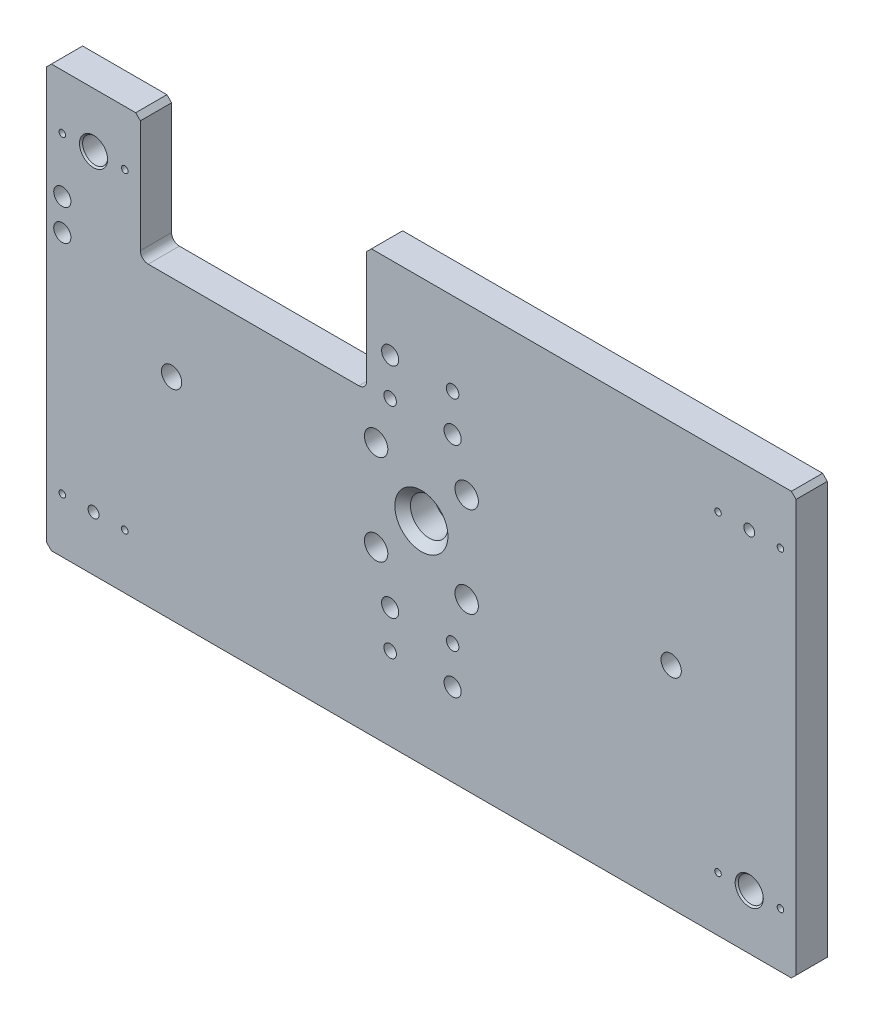
from build123d import *

# Parameters (mm, degrees)
BOSS_EXTRUDE1_DEPTH   = 20
FILLET1_R             = 5
CHAMFER1_SIZE         = 3
HOLE2_D               = 6.6
HOLE2_CBORE_D         = 11
HOLE2_CBORE_DEPTH     = 9
M5_TAPPED_HOLE1_D     = 4.2
M5_TAPPED_HOLE1_DEPTH = 10
M5_TAPPED_HOLE1_TIP   = 1.2618073
M8X1_0_TAPPED_HOLE1_D = 7
HOLE3_D               = 9
HOLE3_CBORE_D         = 16
HOLE3_CBORE_DEPTH     = 12
HOLE4_D               = 9
HOLE4_CBORE_D         = 15
HOLE4_CBORE_DEPTH     = 11
HOLE5_D               = 6.6
HOLE5_CBORE_D         = 11
HOLE5_CBORE_DEPTH     = 9
HOLE6_D               = 8
HOLE7_D               = 24
HOLE8_D               = 13
HOLE8_CBORE_D         = 40
HOLE8_CBORE_DEPTH     = 8
CHAMFER2_SIZE         = 1
CHAMFER3_SIZE         = 5


with BuildPart() as part:
    # Sketch1 → Boss-Extrude1 (new body)
    with BuildSketch(Plane.XY):
        Polygon((18.037295083, 176.592946031), (293.037295083, 176.592946031), (293.037295083, -93.407053969), (-186.962704917, -93.407053969), (-186.962704917, 176.592946031), (-126.962704917, 176.592946031), (-126.962704917, 96.592946031), (18.037295083, 96.592946031), align=None)
    extrude(amount=BOSS_EXTRUDE1_DEPTH)

    # Fillet1
    fillet1_edges = [part.edges().sort_by_distance(p)[0] for p in [
        (-126.962704917, 96.592946031, 10),
        (18.037295083, 96.592946031, 10),
    ]]
    fillet(fillet1_edges, radius=FILLET1_R)

    # Chamfer1
    chamfer1_edges = [part.edges().sort_by_distance(p)[0] for p in [
        (-186.962704917, 176.592946031, 10),
        (-126.962704917, 176.592946031, 10),
        (18.037295083, 176.592946031, 10),
        (293.037295083, 176.592946031, 10),
        (293.037295083, -93.407053969, 10),
        (-186.962704917, -93.407053969, 10),
    ]]
    chamfer(chamfer1_edges, length=CHAMFER1_SIZE)

    # Hole2 (through all)
    with Locations(Plane.XY.offset(20)):
        with Locations((-176.962704917, 106.592946031), (-176.962704917, 86.592946031)):
            CounterBoreHole(HOLE2_D / 2, HOLE2_CBORE_D / 2, HOLE2_CBORE_DEPTH)

    # M5 Tapped Hole1
    with Locations(Plane.XY.offset(20)):
        with Locations((-176.962704917, 141.592946031), (-136.962704917, 141.592946031), (-176.962704917, -58.407053969), (-136.962704917, -58.407053969), (243.037295083, -58.407053969), (283.037295083, -58.407053969), (283.037295083, 141.592946031), (243.037295083, 141.592946031)):
            Hole(M5_TAPPED_HOLE1_D / 2, depth=M5_TAPPED_HOLE1_DEPTH)
            with Locations((0, 0, -(M5_TAPPED_HOLE1_DEPTH + M5_TAPPED_HOLE1_TIP / 2))):  # 118° drill point
                Cone(0, M5_TAPPED_HOLE1_D / 2, M5_TAPPED_HOLE1_TIP, mode=Mode.SUBTRACT)

    # M8x1.0 Tapped Hole1 (through all)
    with Locations(Plane.XY.offset(20)):
        with Locations((-156.962704917, -58.407053969), (263.037295083, 141.592946031)):
            Hole(M8X1_0_TAPPED_HOLE1_D / 2)

    # Hole3 (through all)
    with Locations(Plane.XY.offset(20)):
        with Locations((-156.962704917, 141.592946031), (263.037295083, -58.407053969)):
            CounterBoreHole(HOLE3_D / 2, HOLE3_CBORE_D / 2, HOLE3_CBORE_DEPTH)

    # Hole4 (through all)
    with Locations(Plane.XY.offset(20)):
        with Locations((24.037295083, 70.592946031), (82.037295083, 70.592946031), (82.037295083, 12.592946031), (24.037295083, 12.592946031)):
            CounterBoreHole(HOLE4_D / 2, HOLE4_CBORE_D / 2, HOLE4_CBORE_DEPTH)

    # Hole5 (through all)
    with Locations(Plane.XY.offset(20)):
        with Locations((33.037295083, 123.592946031), (73.037295083, 99.592946031), (33.037295083, -16.407053969), (73.037295083, -40.407053969)):
            CounterBoreHole(HOLE5_D / 2, HOLE5_CBORE_D / 2, HOLE5_CBORE_DEPTH)

    # Hole6 (through all)
    with Locations(Plane.XY.offset(20)):
        with Locations((73.037295083, 123.592946031), (33.037295083, 99.592946031), (33.037295083, -40.407053969), (73.037295083, -16.407053969)):
            Hole(HOLE6_D / 2)

    # Hole7 (through all)
    with Locations(Plane.XY.offset(20)):
        with Locations((53.037295083, 41.592946031)):
            Hole(HOLE7_D / 2)

    # Hole8 (through all)
    with Locations(Plane(origin=(0, 0, 0), x_dir=(-1, 0, 0), z_dir=(0, 0, -1))):
        with Locations((-213.037295083, 41.592946031), (106.962704917, 41.592946031)):
            CounterBoreHole(HOLE8_D / 2, HOLE8_CBORE_D / 2, HOLE8_CBORE_DEPTH)

    # Chamfer2
    chamfer2_edges = [part.edges().sort_by_distance(p)[0] for p in [
        (255.037295083, -58.407053969, 20),
        (-164.962704917, 141.592946031, 20),
        (-86.962704917, 41.592946031, 0),
        (233.037295083, 41.592946031, 0),
    ]]
    chamfer(chamfer2_edges, length=CHAMFER2_SIZE)

    # Chamfer3
    chamfer3_edges = [part.edges().sort_by_distance(p)[0] for p in [
        (65.037295083, 41.592946031, 20),
    ]]
    chamfer(chamfer3_edges, length=CHAMFER3_SIZE)


solid = part.part
